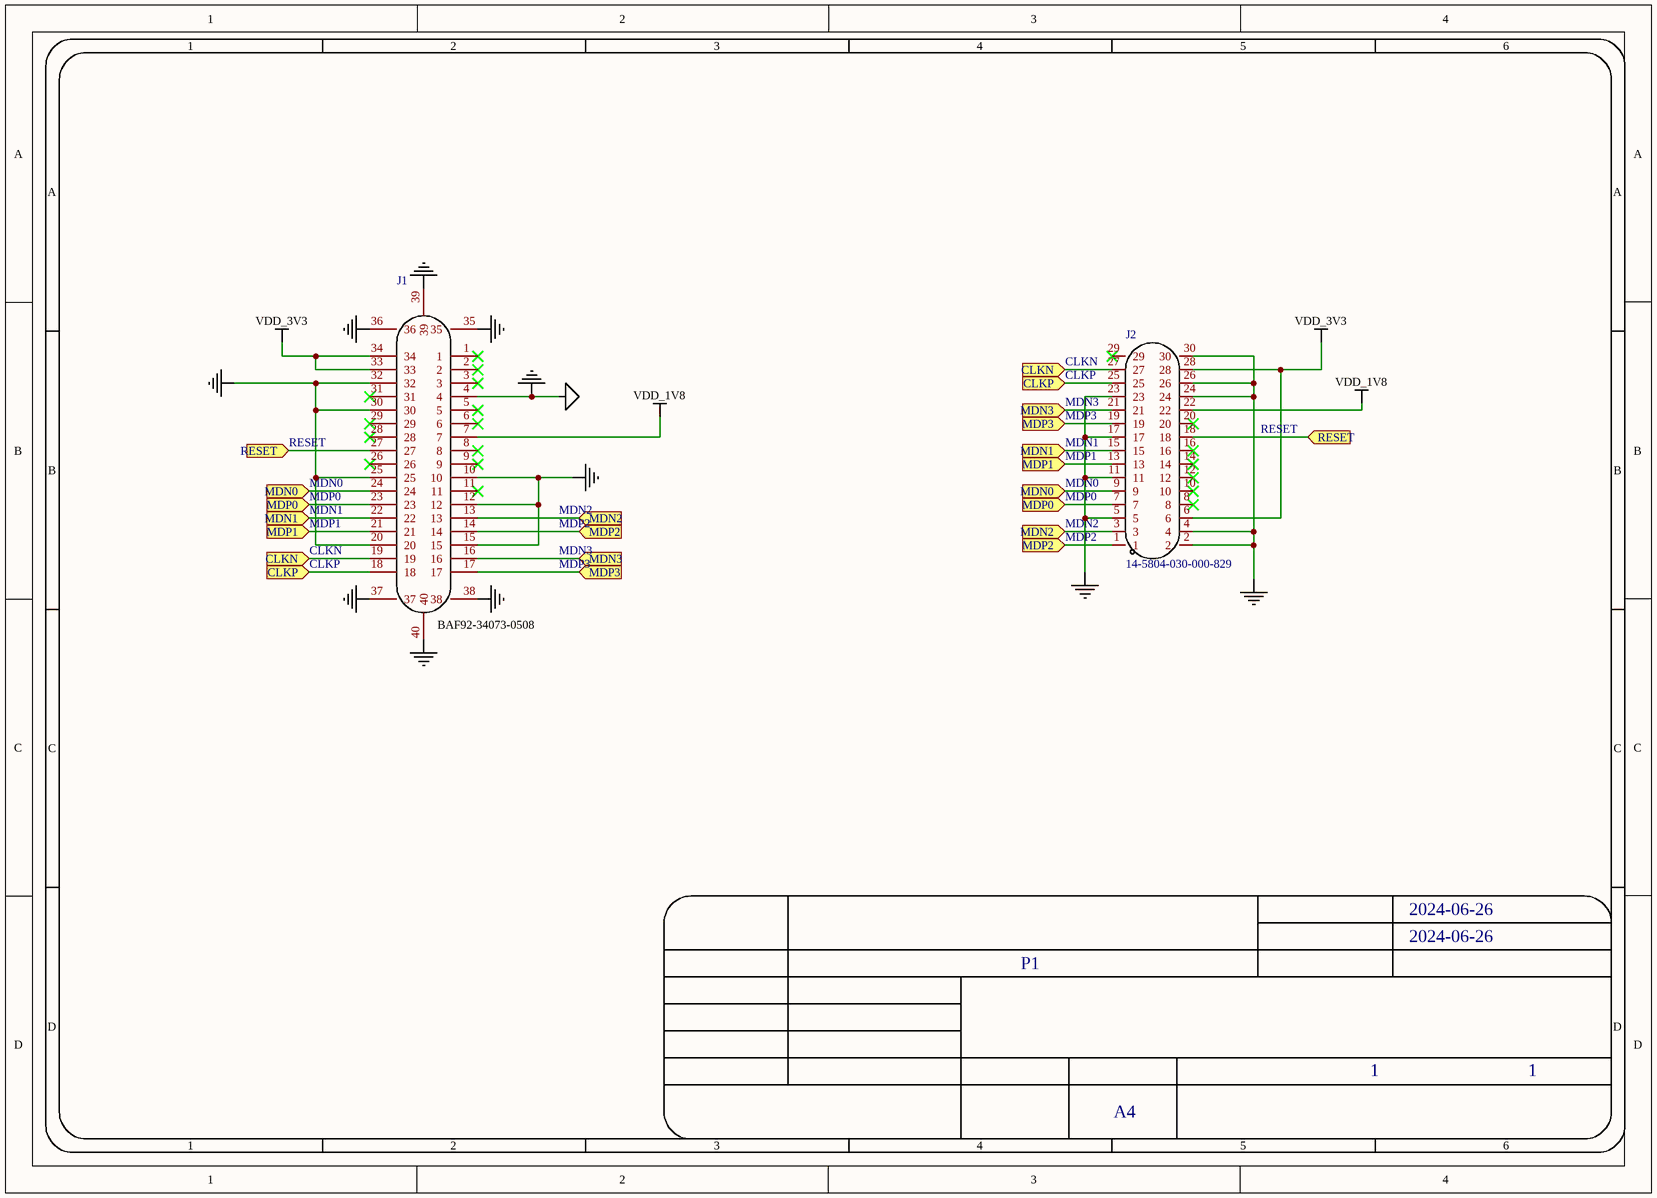
[diagram p0: MISC89352-4.schdoc]
# Altium schematic sheet MISC89352-4.schdoc
size 309 x 223 mm; Version: V1.0; @Project Name: MISC89352; @Page Count: 1; @Update Date: 2024-06-26; @Create Date: 2024-06-26; @Schematic Name: MISC89352; @Page No: 1

## Parts
J1  BAF92-34073-0508  [CONN-SMD_34P-P0.35_BAF92-34073-0508]  (value not drawn)
J2  14-5804-030-000-829  [CONN-SMD_KYOCERA-AVX_145804030020829]

## Ports
CLKN (in), CLKP (in), MDN0 (in), MDN1 (in), MDN2 (in), MDN3 (in), MDP0 (in), MDP1 (in), MDP2 (in), MDP3 (in), RESET (in)

## Nets
AGND: J1.4 J1.10 J1.12 J1.15 J1.20 J1.25 J1.30 J1.32 J1.35 J1.36 J1.37 J1.38 J1.39 J1.40 J2.2 J2.4 J2.5 J2.11 J2.17 J2.23 J2.24 J2.26 J2.30  [also labelled GND]
VDD_1V8: J1.7 J2.22
VDD_3V3: J1.33 J1.34 J2.6 J2.28
CLKN: J1.19 J2.27 ; port CLKN
CLKP: J1.18 J2.25 ; port CLKP
MDN0: J1.24 J2.9 ; port MDN0
MDN1: J1.22 J2.15 ; port MDN1
MDN2: J1.13 J2.3 ; port MDN2
MDN3: J1.16 J2.21 ; port MDN3
MDP0: J1.23 J2.7 ; port MDP0
MDP1: J1.21 J2.13 ; port MDP1
MDP2: J1.14 J2.1 ; port MDP2
MDP3: J1.17 J2.19 ; port MDP3
RESET: J1.27 J2.18 ; port RESET

Not connected (* = marked no-connect by the designer): J1 1* 2* 3* 5* 6* 8* 9* 11* 26* 28* 29* 31*; J2 8* 10* 12* 14* 16* 20* 29*

## Notes on the sheet
- (near J1) BAF92-34073-0508
- 1
- 2
- 3
- 4
- 5
- 6
- A
- B
- C
- 2024-06-26
- P1
- D
- A4

## Library data of the parts
J1 = BAF92-34073-0508: Add into BOM: yes; Symbol: BAF92-34073-0508; Device: BAF92-34073-0508; Convert to PCB: yes
J2 = 14-5804-030-000-829: Add into BOM: yes; Name: 14-5804-030-000-829; Symbol: 14-5804-030-000-829; Device: 14-5804-030-000-829; LCSC Part Name: 14-5804-030-000-829; Supplier Part: C9900008249; Manufacturer Part: 14-5804-030-000-829; Supplier Footprint: CONN-SMD_30P-P0.40; Supplier: LCSC; Convert to PCB: yes